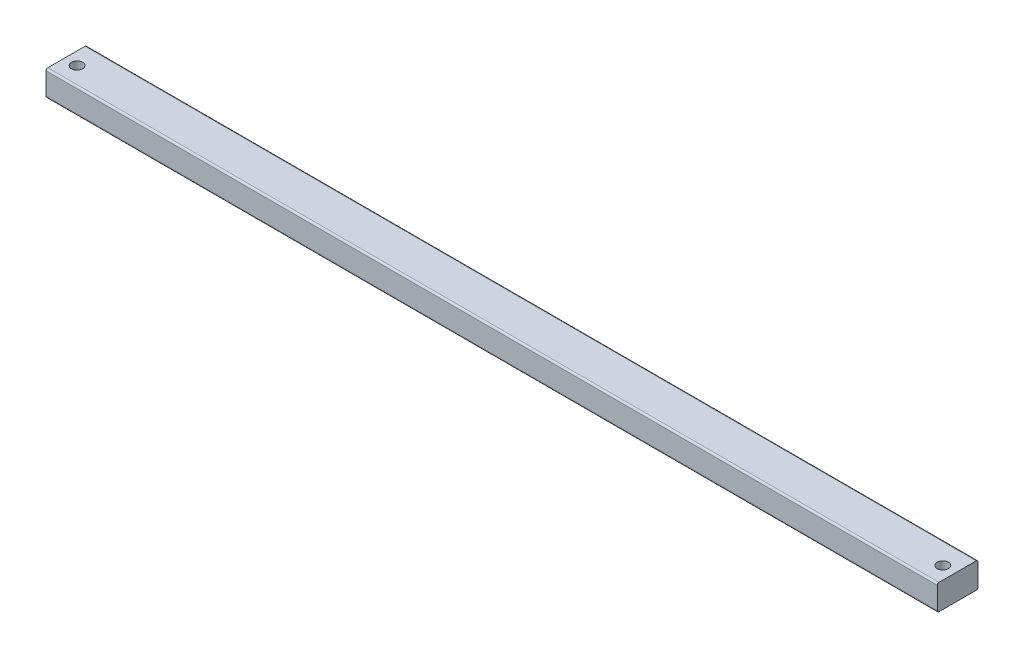
from build123d import *

# Parameters (mm, degrees)
SKETCH2_W          = 40
SKETCH2_H          = 25
FILLET1_R          = 1.7
SKETCH3_R          = 5.5
CUT_EXTRUDE1_DEPTH = 844.414019404


with BuildPart() as part:
    # Sweep1: sweep along a path in Sketch1
    with BuildLine(Plane.XY) as sweep1_path:
        Line((-32.193849021, 0), (842.806150979, 0))
    # Sketch2 → Sweep1 (sweep)
    with BuildSketch(Plane(origin=(-32.193849021, 0, 0), x_dir=(0, 0, -1), z_dir=(1, 0, 0))):
        Rectangle(SKETCH2_W, SKETCH2_H)
    sweep(path=sweep1_path.line)

    # Fillet1
    fillet1_edges = [part.edges().sort_by_distance(p)[0] for p in [
        (405.306150979, 12.5, 20),
        (405.306150979, 12.5, -20),
        (405.306150979, -12.5, -20),
        (405.306150979, -12.5, 20),
    ]]
    fillet(fillet1_edges, radius=FILLET1_R)

    # Sketch3 → Cut-Extrude1 (cut, through all)
    with BuildSketch(Plane(origin=(0, -12.5, 0), x_dir=(-1, 0, 0), z_dir=(0, -1, 0))):
        with Locations(Location((19.693849021, -2, 0), (0, 0, 90))):
            Circle(SKETCH3_R)
        with Locations(Location((-830.306150979, -2, 0), (0, 0, 270))):
            Circle(SKETCH3_R)
    extrude(amount=-CUT_EXTRUDE1_DEPTH, mode=Mode.SUBTRACT)


solid = part.part
